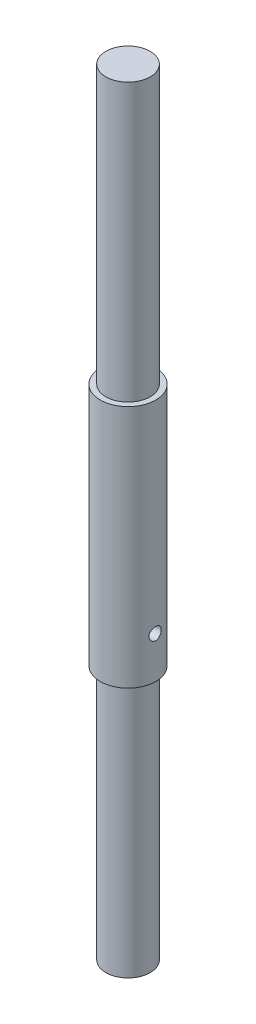
from build123d import *

# Parameters (mm, degrees)
SKETCH_5_R          = 1.1
CUT_EXTRUDE_1_DEPTH = 10


with BuildPart() as part:
    # 草图4 → 旋转1 (revolve)
    with BuildSketch(Plane.XY, mode=Mode.PRIVATE) as revolve_1_sk:
        Polygon((0, 125.008891803), (4, 125.008891803), (4, 75.008891803), (5, 75.008891803), (5, 31.008891803), (4, 31.008891803), (4, -14.991108197), (0, -14.991108197), align=None)
    revolve(revolve_1_sk.sketch.rotate(Axis((0, 0, 0), (0, 1, 0)), 90), axis=Axis((0, 0, 0), (0, 1, 0)))

    # 草图5 → 切除-拉伸1 (cut, symmetric)
    with BuildSketch(Plane(origin=(0, 0, 0), x_dir=(0, 0, -1), z_dir=(1, 0, 0))):
        with Locations((0, 38.508891803)):
            Circle(SKETCH_5_R)
    extrude(amount=CUT_EXTRUDE_1_DEPTH, both=True, mode=Mode.SUBTRACT)


solid = part.part
